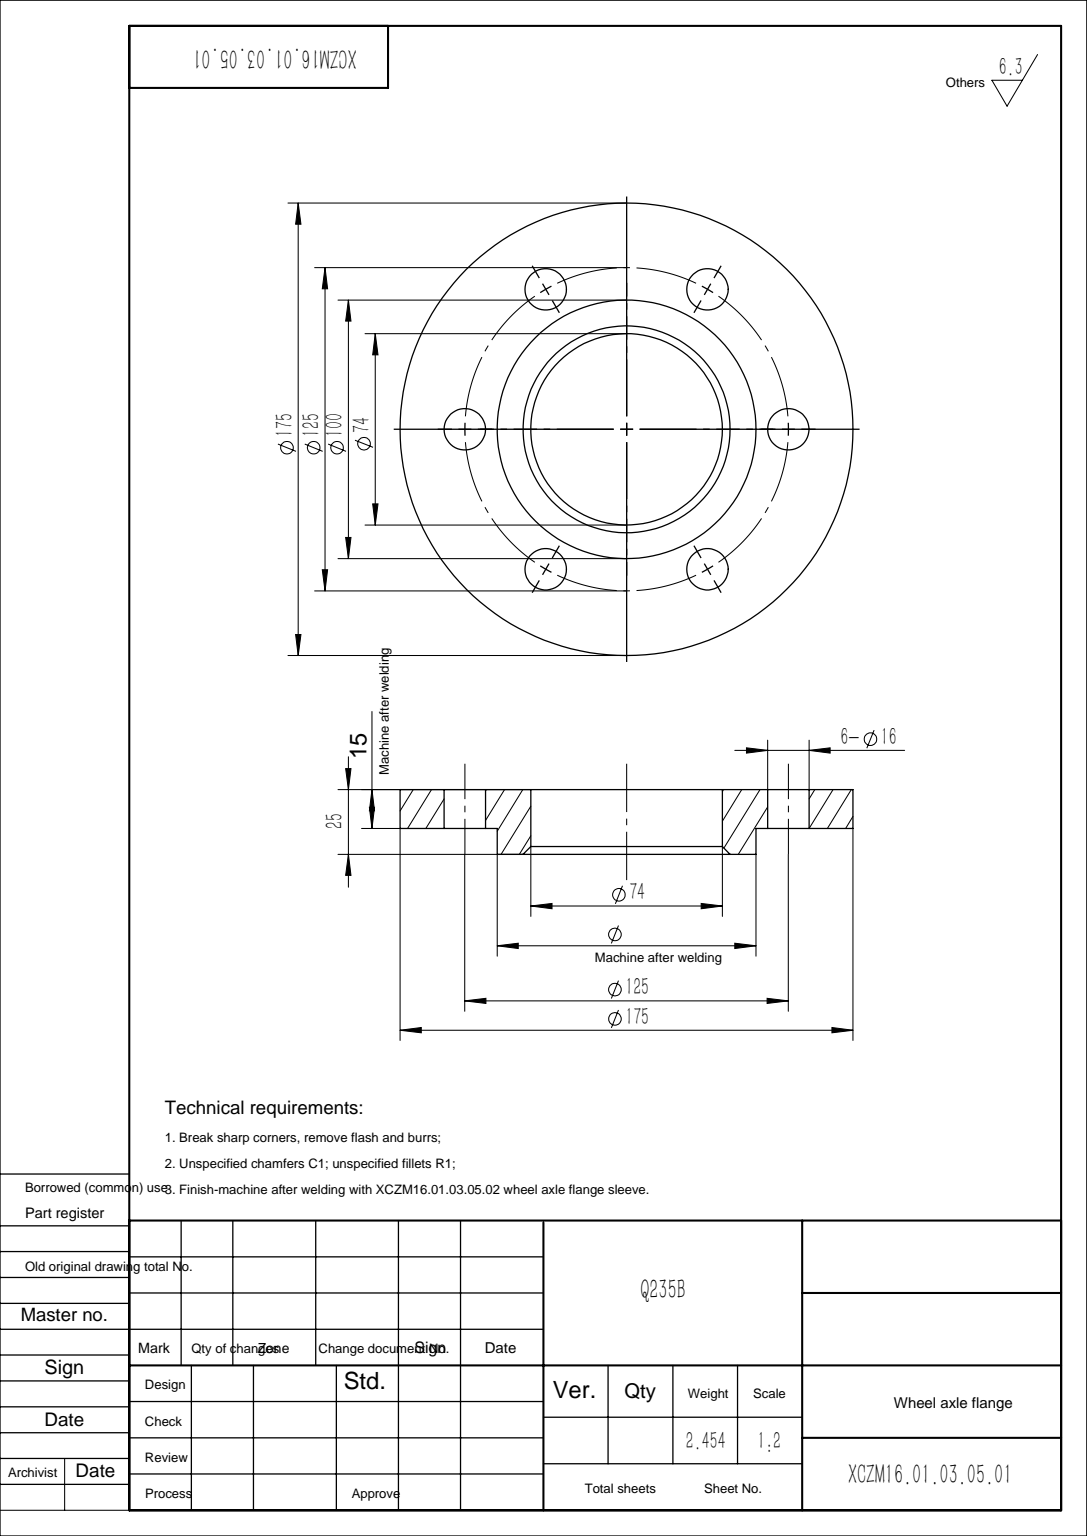
SolidWorks part; units mm, degrees
material "Q235B"
ref_plane "Front Plane" through (0, 0, 0) normal (0, 0, 1) x (1, 0, 0)
ref_plane "Top Plane" through (0, 0, 0) normal (0, 1, 0) x (1, 0, 0)
ref_plane "Right Plane" through (0, 0, 0) normal (1, 0, 0) x (0, 0, -1)
sketch "Sketch1" plane through (0, 0, 0) normal (0, 0, 1) x (1, 0, 0)
  circle A0 centre (0, 0) radius 50
  dimension "D1" = 100
extrude "Boss-Extrude1" add sketch "Sketch1" along normal blind 10
sketch "Sketch2" plane through (0, 0, 0) normal (0, 0, 1) x (1, 0, 0)
  circle A0 centre (0, 0) radius 87.5
  dimension "D1" = 175
extrude "Boss-Extrude2" add sketch "Sketch2" against normal blind 15
sketch "Sketch3" plane through (0, 0, 10) normal (0, 0, 1) x (1, 0, 0)
  circle A0 centre (0, 0) radius 37
  dimension "D1" = 74
extrude "Cut-Extrude1" cut sketch "Sketch3" against normal up to next
hole_wizard "Ø16.0 (16) Diameter Hole1" positions "Sketch4" profile "Sketch5" hole size "Ø16.0" standard "GB" end condition up to next
sketch "Sketch4" plane through (0, 0, 0) normal (0, 0, 1) x (1, 0, 0)
  circle A0 centre (0, 0) radius 62.5
  point P0 (62.5, 0)
  point P13 (31.25, -54.1266)
  point P14 (-31.25, -54.1266)
  point P15 (-62.5, 0)
  point P16 (-31.25, 54.1266)
  point P17 (31.25, 54.1266)
  dimension "D1" = 125
  dimension "D2" = 6
sketch "Sketch5" plane through (62.5, 0, 0) normal (1, 0, 0) x (0, -1, 0)
  line L0 (0, 0) -> (0, 15)
  line L1 (0, 15) -> (8, 15)
  line L2 (8, 15) -> (8, 0)
  line L5 (8, 0) -> (0, 0)
  line L11 (0, -6.35) -> (0, 107.95) construction
  dimension "通孔孔直径" = 16
  dimension "通孔孔深度" = 15
chamfer "Chamfer1" distance 3 angle 45 1 edges at (37, 0, 10)
